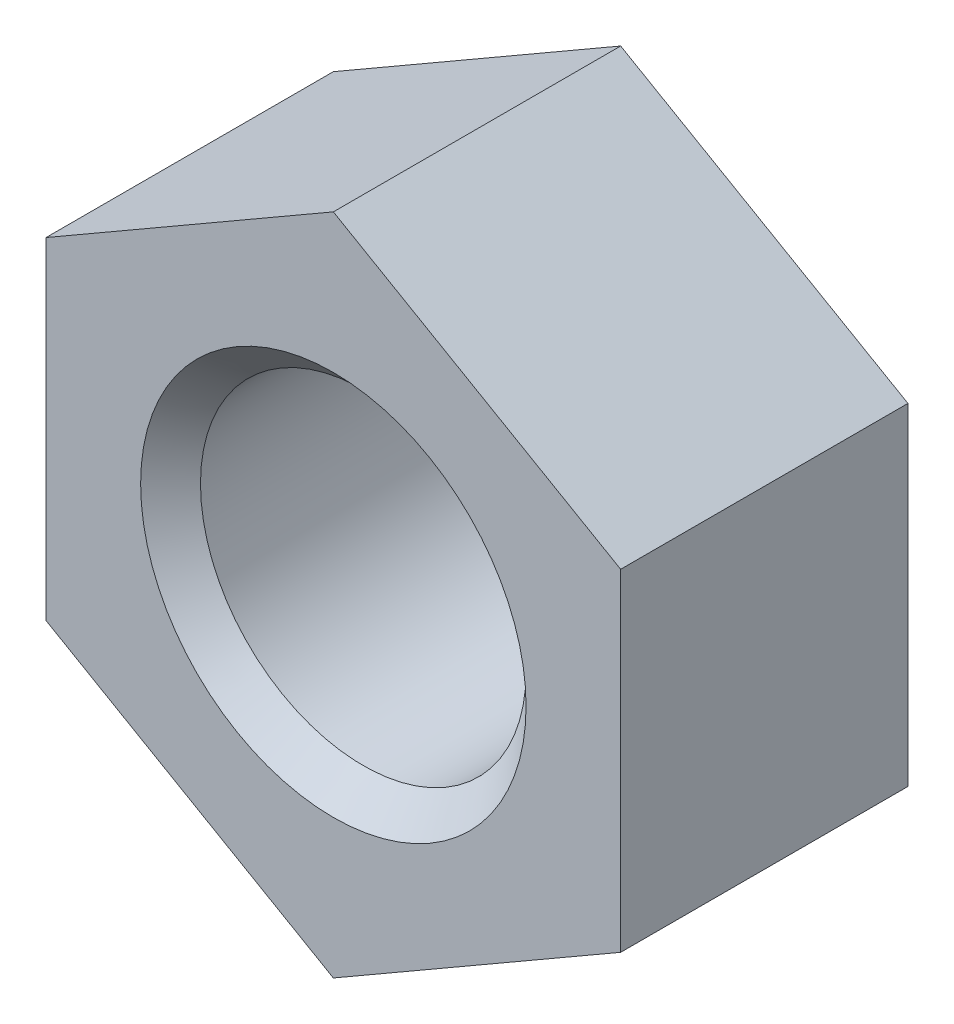
SolidWorks part; units mm, degrees
ref_plane "Front Plane" through (0, 0, 0) normal (0, 0, 1) x (1, 0, 0)
ref_plane "Top Plane" through (0, 0, 0) normal (0, 1, 0) x (1, 0, 0)
ref_plane "Right Plane" through (0, 0, 0) normal (1, 0, 0) x (0, 0, -1)
other "Configuration Table"
sketch "Sketch1" plane through (0, 0, 0) normal (0, 0, 1) x (1, 0, 0)
  line L0 (-5.0939, -2.7153) -> (-5.0939, 4.2129)
  line L1 (-5.0939, 4.2129) -> (0.9061, 7.677)
  line L2 (0.9061, 7.677) -> (6.9061, 4.2129)
  line L3 (6.9061, 4.2129) -> (6.9061, -2.7153)
  line L4 (6.9061, -2.7153) -> (0.9061, -6.1794)
  line L5 (0.9061, -6.1794) -> (-5.0939, -2.7153)
  dimension "D1" = 12
  dimension "D2" = 12
  dimension "D3" = 12
  dimension "D4" = 120
  dimension "D5" = 120
  dimension "D6" = 120
  dimension "D7" = 120
  dimension "D8" = 120
extrude "Boss-Extrude1" add sketch "Sketch1" along normal blind 6
hole_wizard "M8 Tapped Hole1" positions "Sketch2" profile "Sketch3" tap size "M8" standard "GB" end condition through all
sketch "Sketch2" plane through (0, 0, 6) normal (0, 0, 1) x (1, 0, 0)
  line L0 (6.9061, 4.2129) -> (0.9061, 7.677) construction
  line L1 (-5.0939, 4.2129) -> (-5.0939, -2.7153) construction
  line L2 (6.9061, -2.7153) -> (6.9061, 4.2129) construction
  point P0 (0.9061, 0.7488)
  dimension "D1" = 6
  dimension "D2" = 6
  dimension "D3" = 6
sketch "Sketch3" plane through (0.9061, 0.7488, 6) normal (1, 0, 0) x (0, -1, 0)
  line L0 (0, 0) -> (0, 6)
  line L1 (0, 6) -> (3.4, 6)
  line L2 (3.4, 6) -> (3.4, 0.625)
  line L3 (3.4, 0.625) -> (4.025, 0)
  line L5 (4.025, 0) -> (0, 0)
  line L6 (-3.4, 0.625) -> (-4.025, 0) construction
  line L11 (0, -6.35) -> (0, 107.95) construction
  dimension "通孔螺纹孔钻头直径" = 6.8
  dimension "通孔螺纹孔钻头深度" = 6
  dimension "近端锥形沉头孔直径" = 8.05
  dimension "近端锥形沉头孔角度" = 90
cosmetic thread "Cosmetic thread line 1"
